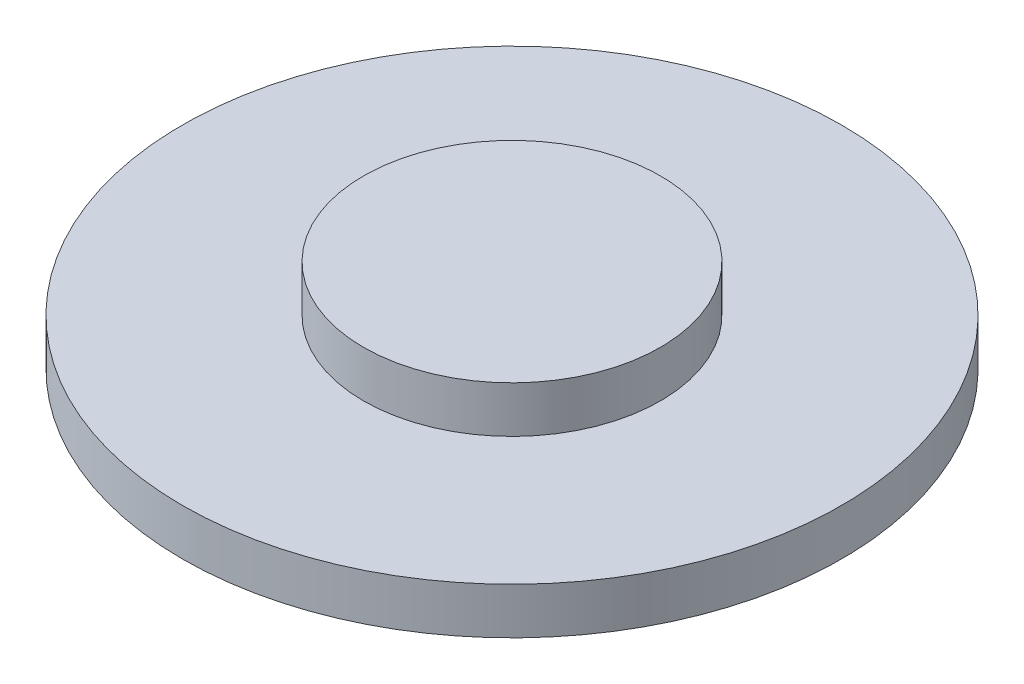
from build123d import *

# Parameters (mm, degrees)
SKETCH1_R           = 35.5
BOSS_EXTRUDE1_DEPTH = 5
SKETCH2_R           = 15.995770756
BOSS_EXTRUDE2_DEPTH = 5


with BuildPart() as part:
    # Sketch1 → Boss-Extrude1 (new body)
    with BuildSketch(Plane(origin=(0, 0, 0), x_dir=(1, 0, 0), z_dir=(0, 1, 0))):
        with Locations(Location((0, 0, 0), (0, 0, 270))):
            Circle(SKETCH1_R)
    extrude(amount=BOSS_EXTRUDE1_DEPTH)

    # Sketch2 → Boss-Extrude2 (add)
    with BuildSketch(Plane(origin=(0, 5, 0), x_dir=(1, 0, 0), z_dir=(0, 1, 0))):
        with Locations(Location((0, 0, 0), (0, 0, 270))):
            Circle(SKETCH2_R)
    extrude(amount=BOSS_EXTRUDE2_DEPTH)


solid = part.part
